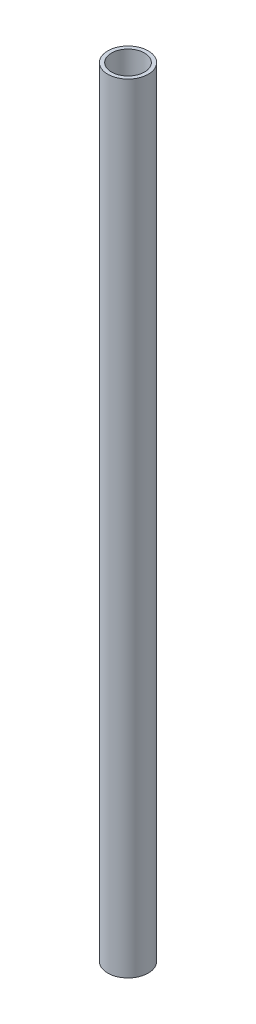
from build123d import *

# Parameters (mm, degrees)
SKETCH1_R                              = 38
SKETCH1_R_2                            = 31
GB_T_6728_2002_ROUND_TUBE_76_7_1_DEPTH = 1460


with BuildPart() as part:
    # Sketch1 → Gb/t 6728-2002 round tube 76×7(1) (new body)
    with BuildSketch(Plane(origin=(0, 0, 0), x_dir=(-1, 0, 0), z_dir=(0, 1, 0))):
        Circle(SKETCH1_R)
        Circle(SKETCH1_R_2, mode=Mode.SUBTRACT)
    extrude(amount=GB_T_6728_2002_ROUND_TUBE_76_7_1_DEPTH)


solid = part.part
